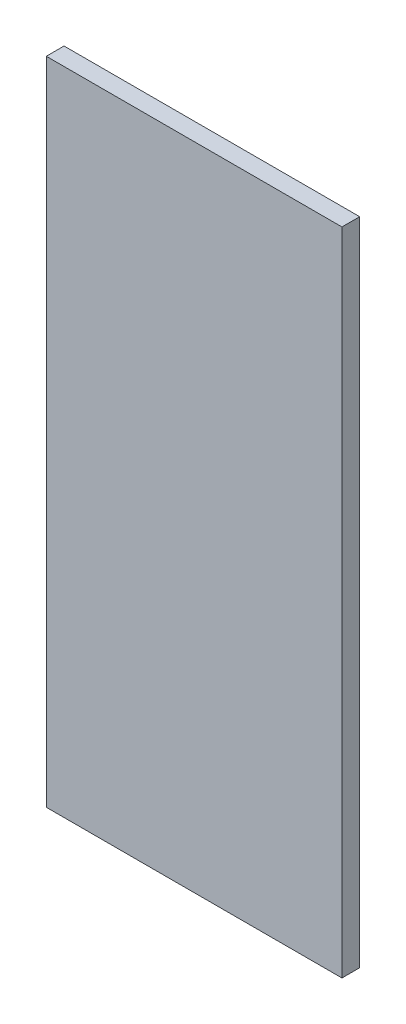
SolidWorks part; units mm, degrees
ref_plane "前视基准面" through (0, 0, 0) normal (0, 0, 1) x (1, 0, 0)
ref_plane "上视基准面" through (0, 0, 0) normal (0, 1, 0) x (1, 0, 0)
ref_plane "右视基准面" through (0, 0, 0) normal (1, 0, 0) x (0, 0, -1)
sketch "草图1" plane through (0, 0, 0) normal (0, 0, 1) x (1, 0, 0)
  line L1 (-50, 110) -> (50, 110)
  line L2 (-50, 110) -> (-50, -110)
  line L3 (-50, -110) -> (50, -110)
  line L4 (50, 110) -> (50, -110)
  line L5 (-50, 110) -> (50, -110) construction
  line L6 (-50, -110) -> (50, 110) construction
  point P0 (0, 0)
  dimension "D1" = 220
  dimension "D2" = 100
extrude "凸台-拉伸1" add sketch "草图1" along normal blind 6
